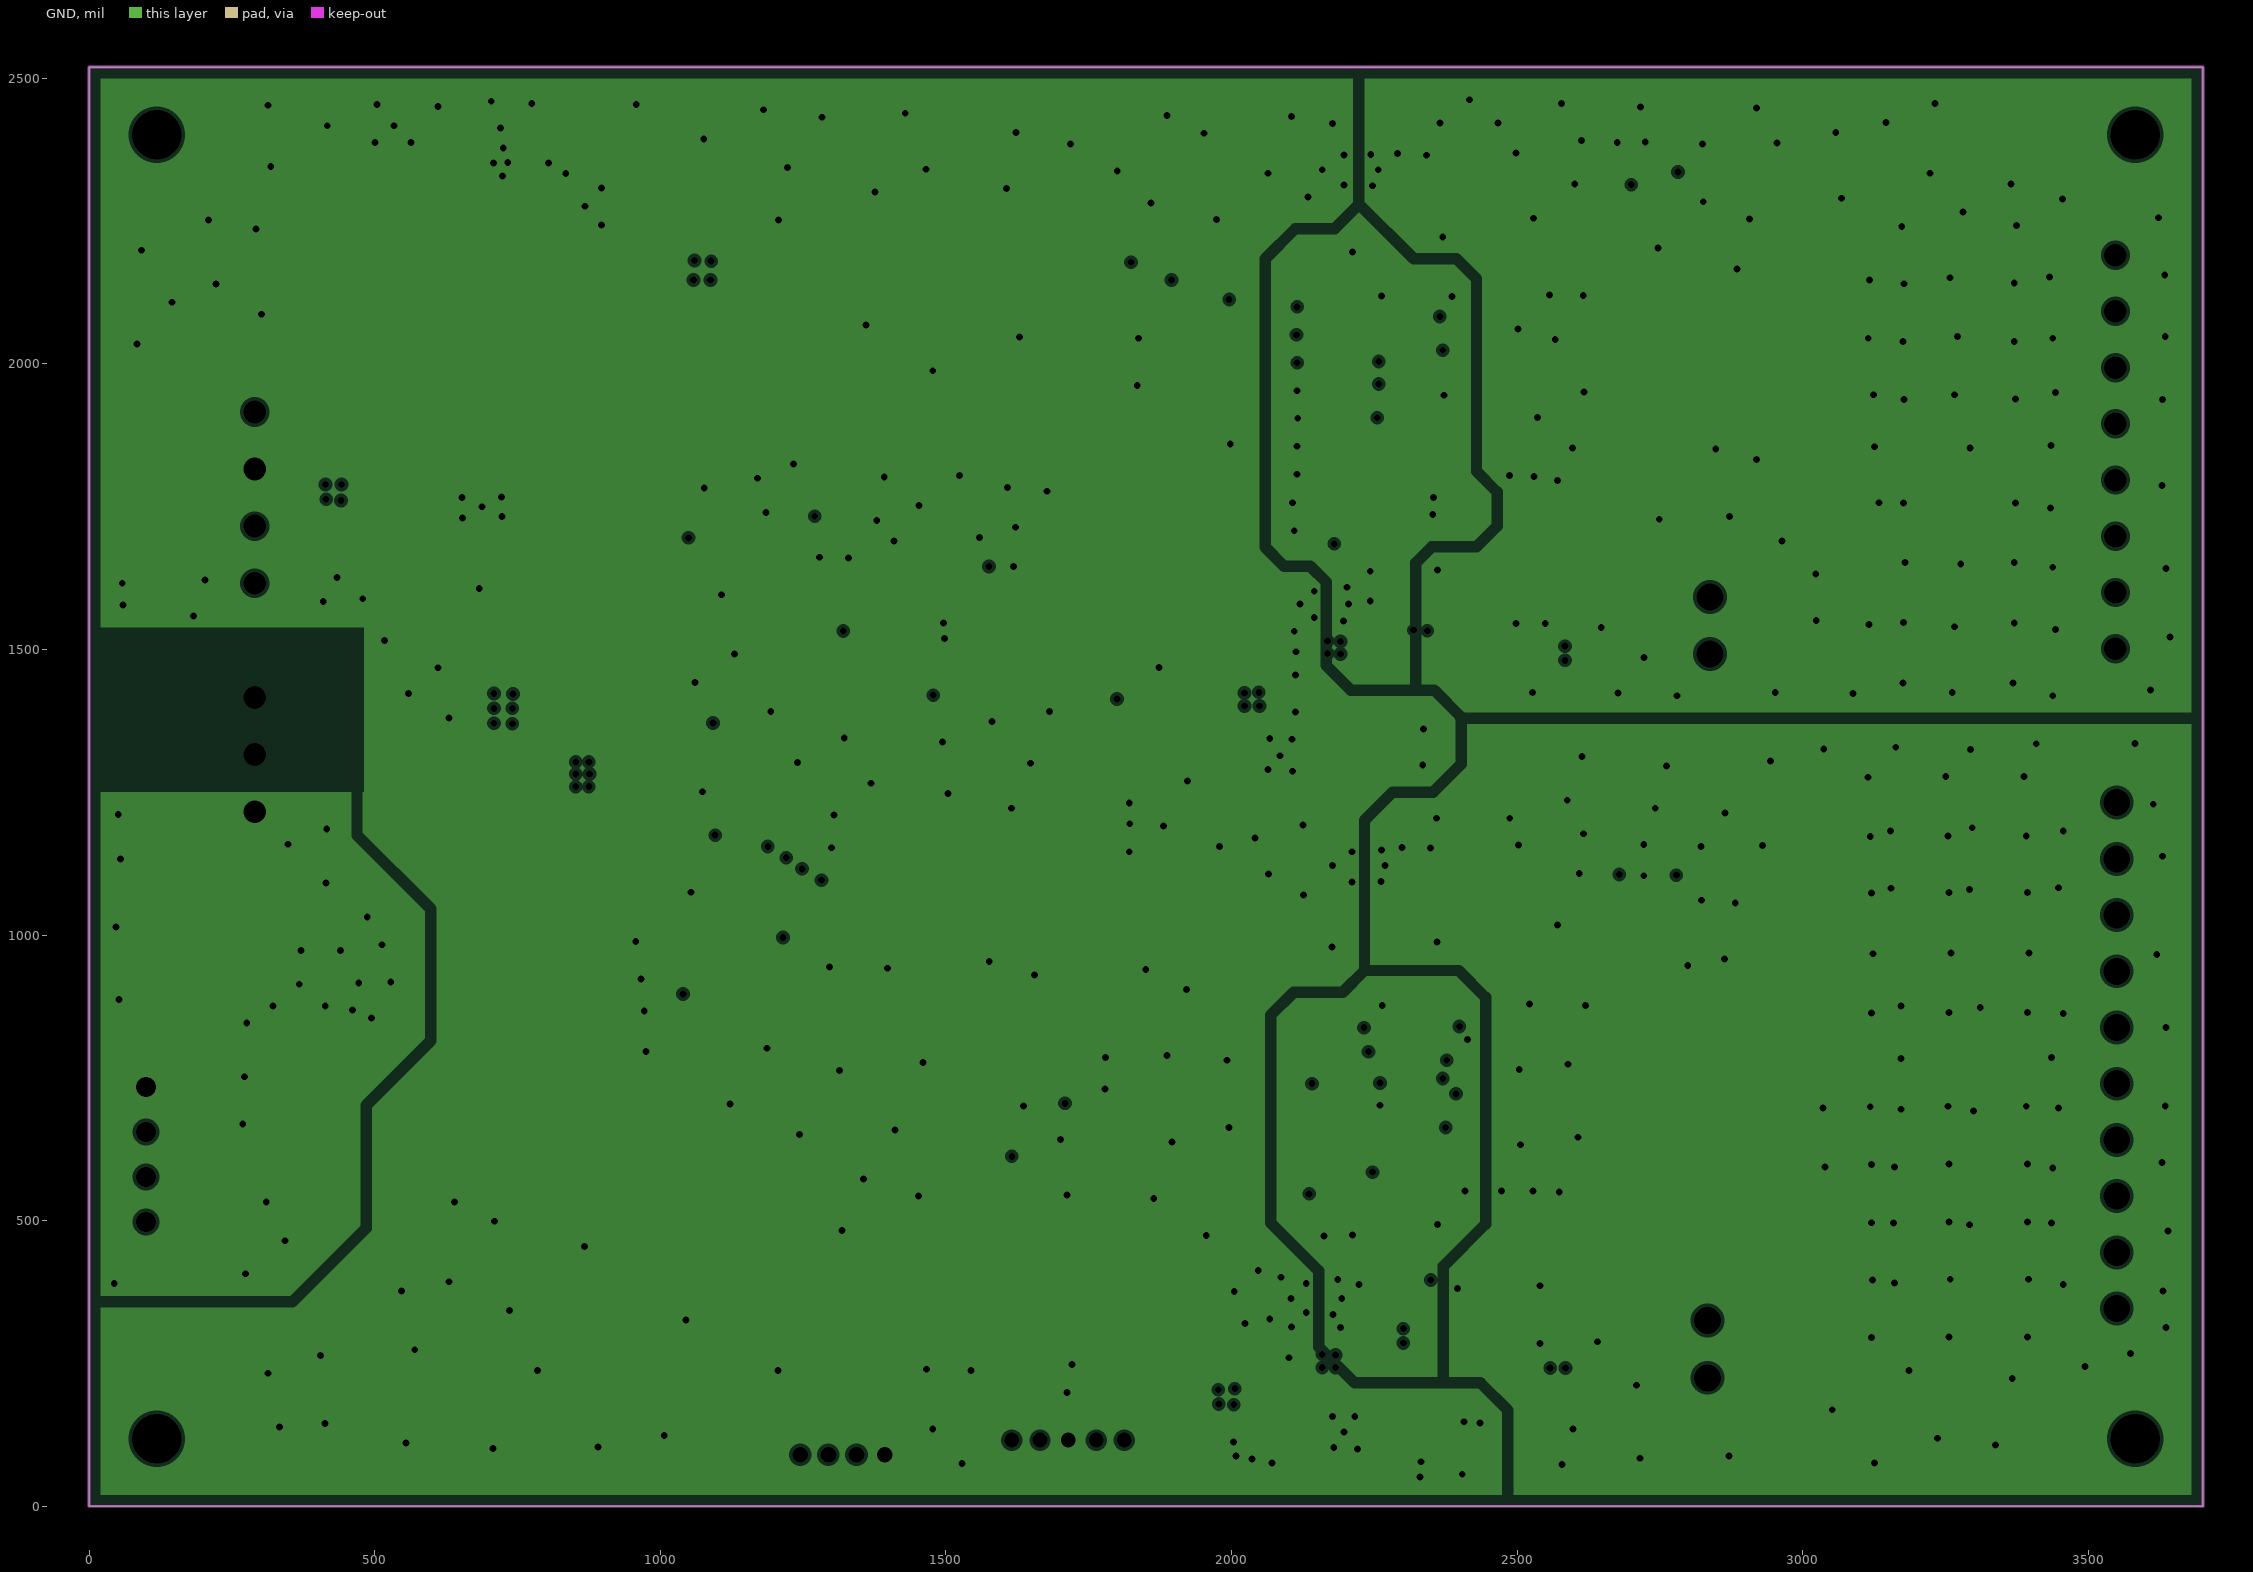
[diagram p0: GND, clearances drawn from the general rule]
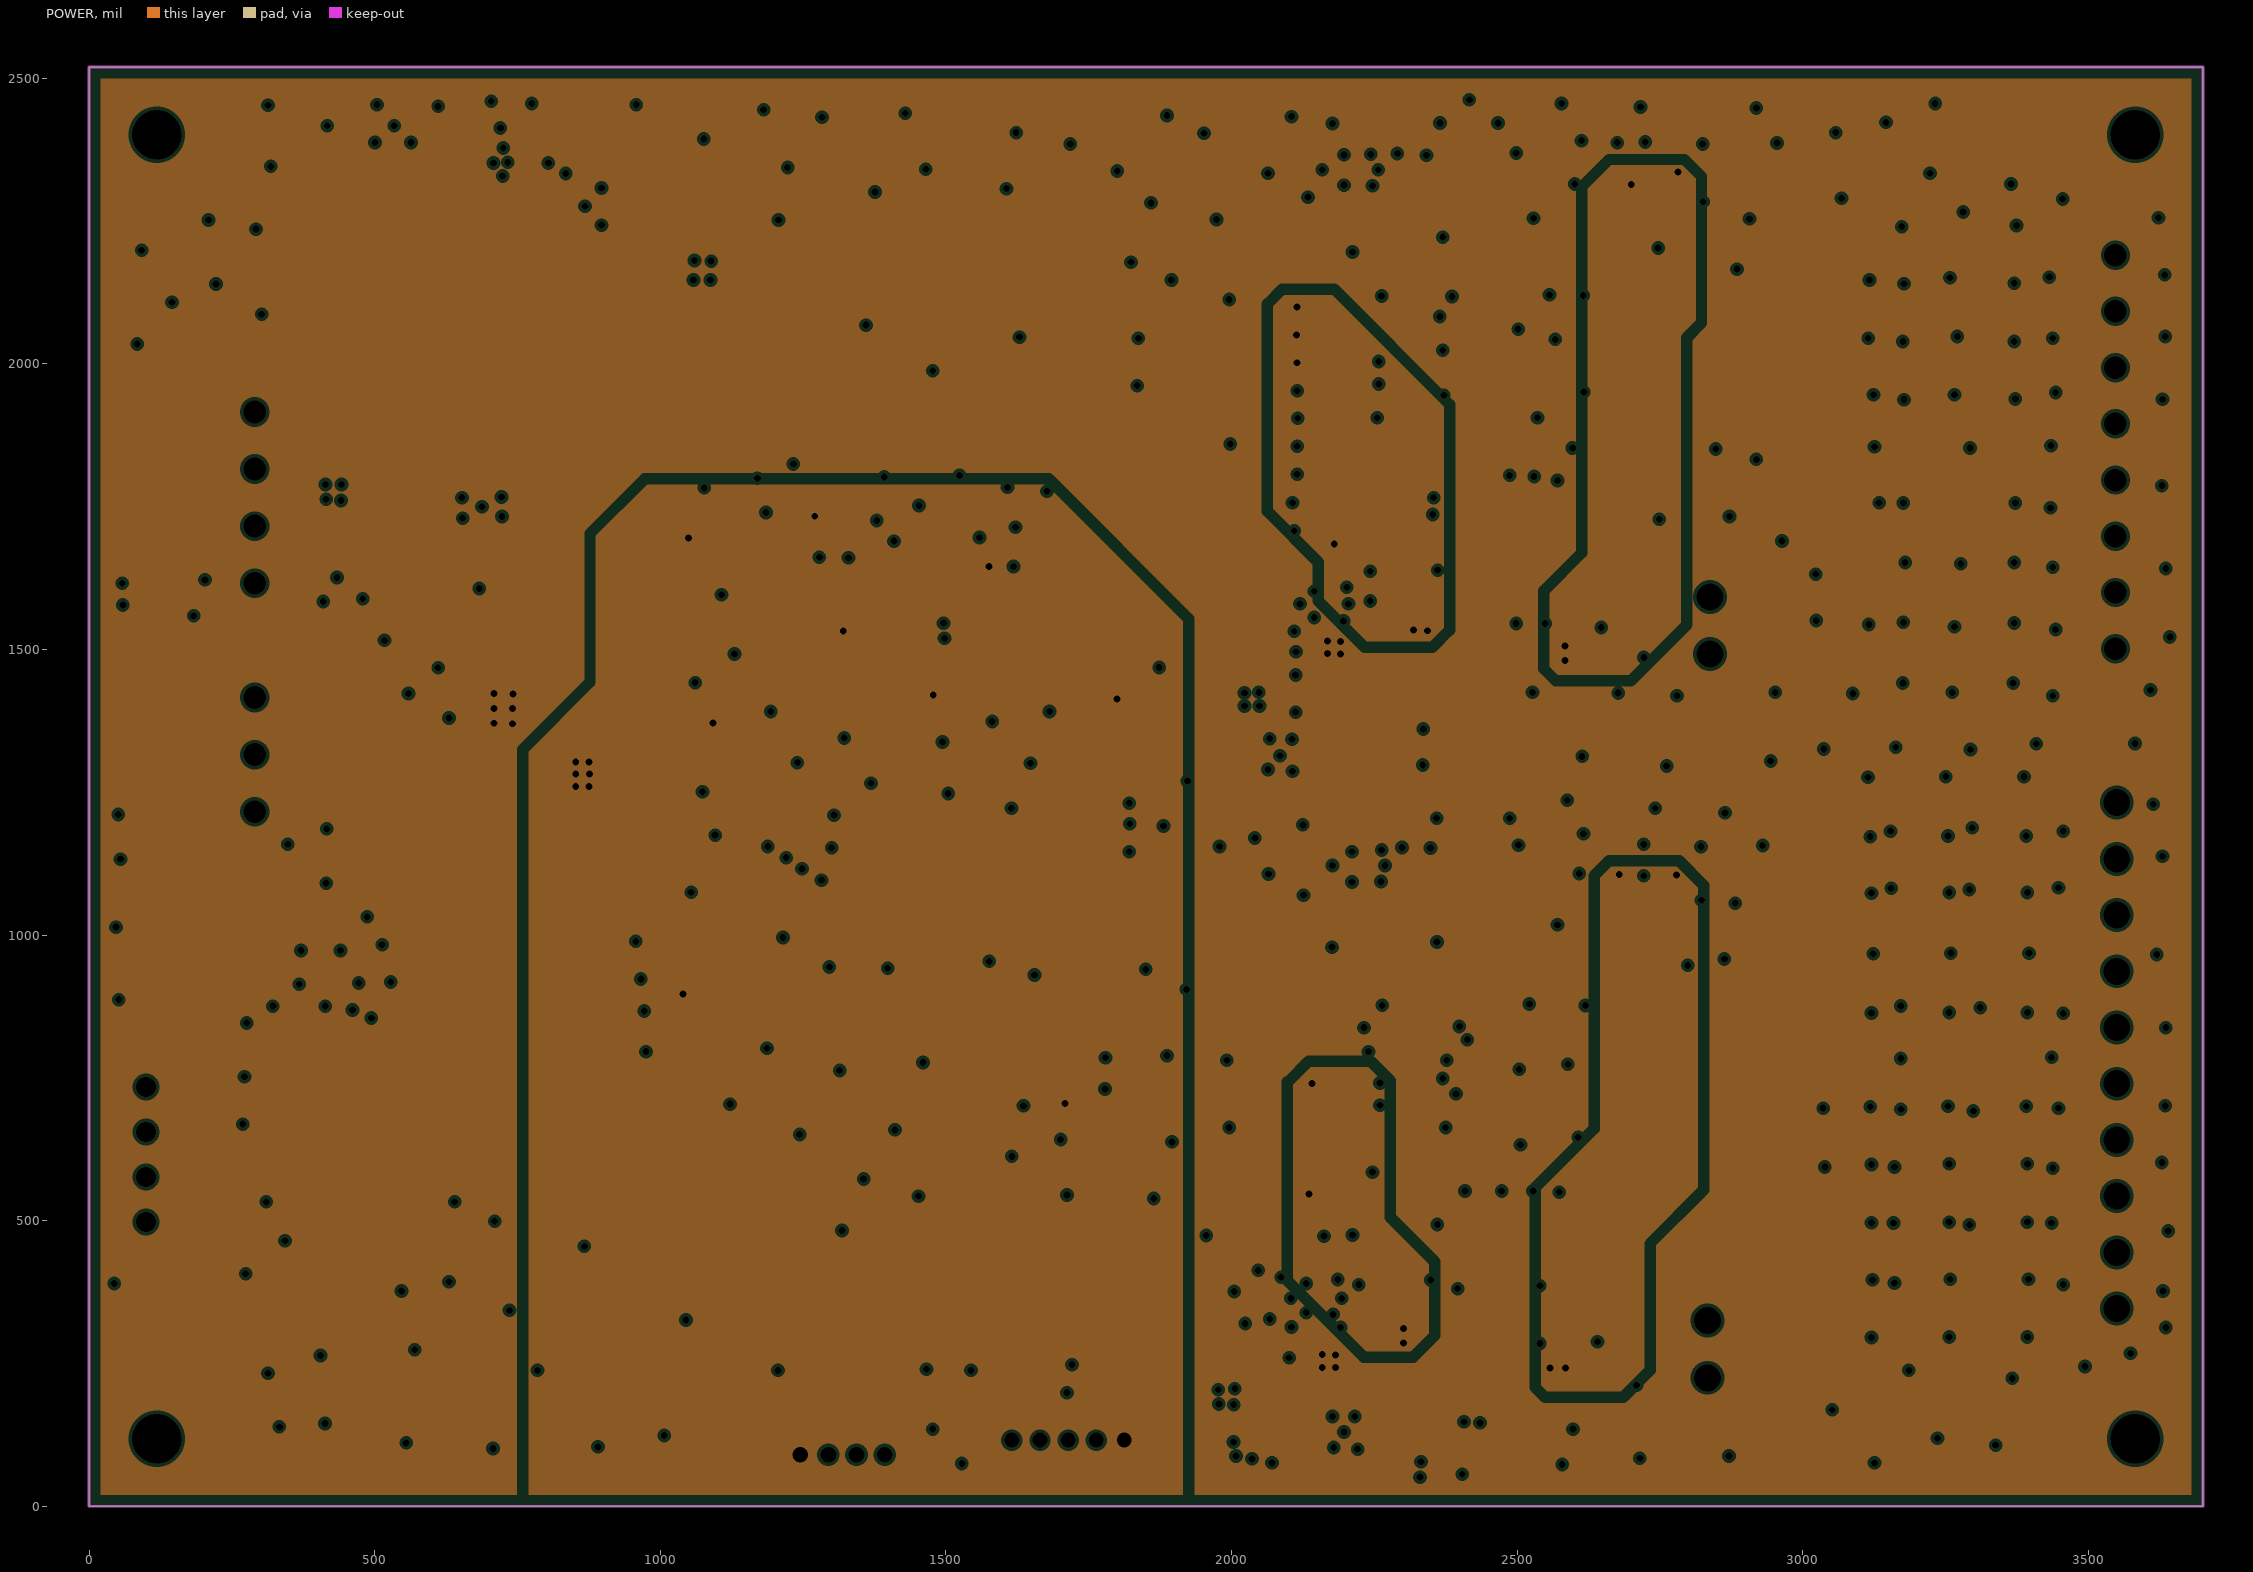
[diagram p1: POWER, clearances drawn from the general rule]
# Altium PCB MISC86293.PcbDoc (part 2 of 4)
## Footprints (in the part's own frame and the unit in brackets; to place one, negate y for a bottom-side part, rotate by r counter-clockwise, add the part's x,y. Pads: shape width x height; smd on the part's side, far side on the other; paste and mask are expansions set on the pad) (continued)
CAP-SMD_L3.2-W1.6 [mm]
  rect 1.2x1.4 smd: 1(-1.35,0) 2(1.35,0)
  silkscreen extent -1.6,-1.14 1.6,1.14
CONN-TH_4P-P1.25_WAFER-MX1.25-4PZZ [mm]
  rect 0.9x1.5 hole 0.7 paste+0 mask+0.05: 1(1.875,0) 2(0.625,0) 3(-0.625,0) 4(-1.875,0)
  silkscreen extent -3.43,-2.02 3.43,1.21
CONN-TH_5P-P1.25_XUNPU_WAFER-MX1.25-5PZZ [mm]
  rect 1x0.9 hole 0.65: 1(-2.5,0)
  round 1 hole 0.65: 2(-1.25,0) 3(0,0) 4(1.25,0) 5(2.5,0)
  silkscreen extent -4.07,-2.03 4.07,1.27
CONN-TH_A2001WV-4P [mm]
  round 1.5 hole 0.9 paste+0 mask+0.05: 1(3,0) 2(1,0) 3(-1,0) 4(-3,0)
  silkscreen extent -5,-1.8 5,2.7
CONN-TH_A2501WV-10P [mm]
  round 1.8 hole 1.2: 1(11.25,0) 2(8.75,0) 3(6.25,0) 4(3.75,0) 5(1.25,0) 6(-1.25,0) 7(-3.75,0) 8(-6.25,0) 9(-8.75,0) 10(-11.25,0)
  silkscreen extent -13.88,-2.38 13.82,3.5
CONN-TH_WF-1A254A8P [mm]
  round 1.6 hole 1: 1(-8.75,0) 2(-6.25,0) 3(-3.75,0) 4(-1.25,0) 5(1.25,0) 6(3.75,0) 7(6.25,0) 8(8.75,0)
  silkscreen extent -11.25,-2.35 11.25,3.55
CRYSTAL-SMD_4P-L3.2-W2.5-BL [mm]
  rect 1.4x1.2 smd: 1(-1.1,-0.85) 2(1.1,-0.85) 3(1.1,0.85) 4(-1.1,0.85)
  silkscreen extent -2.26,-1.91 2.03,1.68
HDR-TH_2P-P2.54-V-M [mm]
  rect 2x2 hole 1.2: 1(-1.27,0)
  round 2 hole 1.2: 2(1.27,0)
  silkscreen extent -2.54,-1.27 2.54,1.27
IND-SMD_L4.0-W4.0_FNR40XXS [mm]
  rect 1.6x3.9 smd: 1(-1.5,0) 2(1.5,0)
  silkscreen extent -2,-2.1 2,2.1
L0402 [mm]
  rect 0.79x0.54 smd paste-100 mask+0.051: 1(-0.545,0) 2(0.545,0)
  silkscreen extent -1.17,-0.5 1.17,0.5
L0603 [mm]
  rect 0.8x0.864 smd paste-100 mask+0.051: 1(-0.7,0) 2(0.7,0)
  silkscreen extent -1.42,-0.65 1.41,0.67
LED0603-RD [mm]
  rect 0.8x0.8 smd: 1(-0.799,0) 2(0.799,0)
  silkscreen extent -1.49,-0.75 1.39,0.76
LQFP-100_L14.0-W14.0-P0.50-LS16.0-BL [mm]
  oval 0.3x1.6 smd paste-100 mask+0.051: 1(-6,-7.55) 2(-5.5,-7.55) 3(-5,-7.55) 4(-4.5,-7.55) 5(-4,-7.55) 6(-3.5,-7.55) 7(-3,-7.55) 8(-2.5,-7.55) 9(-2,-7.55) 10(-1.5,-7.55) 11(-1,-7.55) 12(-0.5,-7.55) 13(0,-7.55) 14(0.5,-7.55) 15(1,-7.55) 16(1.5,-7.55) 17(2,-7.55) 18(2.5,-7.55) 19(3,-7.55) 20(3.5,-7.55) 21(4,-7.55) 22(4.5,-7.55) 23(5,-7.55) 24(5.5,-7.55) 25(6,-7.55) 51(6,7.55) 52(5.5,7.55) 53(5,7.55) 54(4.5,7.55) 55(4,7.55) 56(3.5,7.55) 57(3,7.55) 58(2.5,7.55) 59(2,7.55) 60(1.5,7.55) 61(1,7.55) 62(0.5,7.55) 63(0,7.55) 64(-0.5,7.55) 65(-1,7.55) 66(-1.5,7.55) 67(-2,7.55) 68(-2.5,7.55) 69(-3,7.55) 70(-3.5,7.55) 71(-4,7.55) 72(-4.5,7.55) 73(-5,7.55) 74(-5.5,7.55) 75(-6,7.55)
  oval 1.6x0.3 smd paste-100 mask+0.051: 26(7.55,-6) 27(7.55,-5.5) 28(7.55,-5) 29(7.55,-4.5) 30(7.55,-4) 31(7.55,-3.5) 32(7.55,-3) 33(7.55,-2.5) 34(7.55,-2) 35(7.55,-1.5) 36(7.55,-1) 37(7.55,-0.5) 38(7.55,0) 39(7.55,0.5) 40(7.55,1) 41(7.55,1.5) 42(7.55,2) 43(7.55,2.5) 44(7.55,3) 45(7.55,3.5) 46(7.55,4) 47(7.55,4.5) 48(7.55,5) 49(7.55,5.5) 50(7.55,6) 76(-7.55,6) 77(-7.55,5.5) 78(-7.55,5) 79(-7.55,4.5) 80(-7.55,4) 81(-7.55,3.5) 82(-7.55,3) 83(-7.55,2.5) 84(-7.55,2) 85(-7.55,1.5) 86(-7.55,1) 87(-7.55,0.5) 88(-7.55,0) 89(-7.55,-0.5) 90(-7.55,-1) 91(-7.55,-1.5) 92(-7.55,-2) 93(-7.55,-2.5) 94(-7.55,-3) 95(-7.55,-3.5) 96(-7.55,-4) 97(-7.55,-4.5) 98(-7.55,-5) 99(-7.55,-5.5) 100(-7.55,-6)
  silkscreen extent -7.03,-8 6.25,6.25
MSOP-10_L3.0-W3.0-P0.50-LS5.0-BL-EP [mm]
  oval 0.28x1.62 smd paste-100 mask+0.051: 1(-1,-2.11) 2(-0.5,-2.11) 3(0,-2.11) 4(0.5,-2.11) 5(1,-2.11) 6(1,2.11) 7(0.5,2.11) 8(0,2.11) 9(-0.5,2.11) 10(-1,2.11)
  rect 2.1x1.83 smd paste-100 mask+0.051: 11(0,0)
  silkscreen extent -1.84,-2.35 1.52,1.52
MSOP-12_L4.0-W3.0-P0.65-LS4.9-BL-EP [mm]
  rect 0.3x1.3 smd paste+0.051 mask+0: 1(-1.625,-2.375) 2(-0.975,-2.375) 3(-0.325,-2.375) 4(0.325,-2.375) 5(0.975,-2.375) 6(1.625,-2.375)
  rect 0.35x1.3 smd paste+0.051 mask+0: 7(1.625,2.375) 8(0.975,2.375) 9(0.325,2.375) 10(-0.325,2.375) 11(-0.975,2.375) 12(-1.625,2.375)
  rect 2.85x1.65 smd paste+0.051 mask+0: 13(0,-0.038)
  silkscreen extent -2.51,-2.3 1.98,1.45
PWRM-TH_WRA0512S-3WR2 [mil]
  round 70 hole 40 paste+2 mask+0: 1(-350,0) 2(-250,0) 3(-150,0) 5(50,0) 6(150,0) 7(250,0) 8(350,0)
  silkscreen extent -433,-276 433,98
R0402 [mm]
  rect 0.566x0.54 smd paste-100 mask+0.051: 1(-0.433,0) 2(0.433,0)
  silkscreen extent -0.94,-0.5 0.94,0.5
R0603 [mil]
  rect 31.75x34.02 smd paste-3937.01 mask+2: 1(-29.66,0) 2(29.66,0)
  silkscreen extent -55,-26 55,26
SMA_L4.3-W2.6-LS5.2-RD [mm]
  rect 2x2 smd: 1(-2.2,0) 2(2.2,0)
  silkscreen extent -2.98,-1.5 2.6,1.5
SOIC-8_L4.9-W3.9-P1.27-LS6.0-BL [mm]
  oval 0.588x2.045 smd: 1(-1.905,-2.772) 2(-0.635,-2.772) 3(0.635,-2.772) 4(1.905,-2.772) 5(1.905,2.772) 6(0.635,2.772) 7(-0.635,2.772) 8(-1.905,2.772)
  silkscreen extent -2.8,-2.92 2.53,1.52
SOT-23-3_L2.9-W1.3-P1.90-LS2.4-BR [mm]
  rect 1.25x0.7 smd: 1(1,-0.95) 2(1,0.95) 3(-1,0)
  silkscreen extent -0.73,-1.53 0.73,1.53
SOT-23-5_L3.0-W1.7-P0.95-LS2.8-BR [mm]
  rect 1.1x0.6 smd: 1(1.3,-0.95) 2(1.3,0) 3(1.3,0.95) 4(-1.3,0.95) 5(-1.3,-0.95)
  silkscreen extent -0.9,-1.78 1.65,1.55
SW-SMD_L3.9-W3.0-P4.45 [mm]
  rect 1.23x1.36 smd: 1(-2.185,0) 2(2.185,0)
  silkscreen extent -2.03,-1.62 2.25,1.62
TQFP-64_L10.0-W10.0-P0.50-LS12.0-BL [mm]
  oval 0.28x1.8 smd: 1(-3.75,-5.55) 2(-3.25,-5.55) 3(-2.75,-5.55) 4(-2.25,-5.55) 5(-1.75,-5.55) 6(-1.25,-5.55) 7(-0.75,-5.55) 8(-0.25,-5.55) 9(0.25,-5.55) 10(0.75,-5.55) 11(1.25,-5.55) 12(1.75,-5.55) 13(2.25,-5.55) 14(2.75,-5.55) 15(3.25,-5.55) 16(3.75,-5.55) 33(3.75,5.55) 34(3.25,5.55) 35(2.75,5.55) 36(2.25,5.55) 37(1.75,5.55) 38(1.25,5.55) 39(0.75,5.55) 40(0.25,5.55) 41(-0.25,5.55) 42(-0.75,5.55) 43(-1.25,5.55) 44(-1.75,5.55) 45(-2.25,5.55) 46(-2.75,5.55) 47(-3.25,5.55) 48(-3.75,5.55)
  oval 1.8x0.28 smd: 17(5.55,-3.75) 18(5.55,-3.25) 19(5.55,-2.75) 20(5.55,-2.25) 21(5.55,-1.75) 22(5.55,-1.25) 23(5.55,-0.75) 24(5.55,-0.25) 25(5.55,0.25) 26(5.55,0.75) 27(5.55,1.25) 28(5.55,1.75) 29(5.55,2.25) 30(5.55,2.75) 31(5.55,3.25) 32(5.55,3.75) 49(-5.55,3.75) 50(-5.55,3.25) 51(-5.55,2.75) 52(-5.55,2.25) 53(-5.55,1.75) 54(-5.55,1.25) 55(-5.55,0.75) 56(-5.55,0.25) 57(-5.55,-0.25) 58(-5.55,-0.75) 59(-5.55,-1.25) 60(-5.55,-1.75) 61(-5.55,-2.25) 62(-5.55,-2.75) 63(-5.55,-3.25) 64(-5.55,-3.75)
  silkscreen extent -5.4,-7.04 5,5
TQFP-64_L10.0-W10.0-P0.50-LS12.0-TL [mm]
  oval 1.8x0.28 smd paste-100 mask+0.051: 1(-5.55,3.75) 2(-5.55,3.25) 3(-5.55,2.75) 4(-5.55,2.25) 5(-5.55,1.75) 6(-5.55,1.25) 7(-5.55,0.75) 8(-5.55,0.25) 9(-5.55,-0.25) 10(-5.55,-0.75) 11(-5.55,-1.25) 12(-5.55,-1.75) 13(-5.55,-2.25) 14(-5.55,-2.75) 15(-5.55,-3.25) 16(-5.55,-3.75) 33(5.55,-3.75) 34(5.55,-3.25) 35(5.55,-2.75) 36(5.55,-2.25) 37(5.55,-1.75) 38(5.55,-1.25) 39(5.55,-0.75) 40(5.55,-0.25) 41(5.55,0.25) 42(5.55,0.75) 43(5.55,1.25) 44(5.55,1.75) 45(5.55,2.25) 46(5.55,2.75) 47(5.55,3.25) 48(5.55,3.75)
  oval 0.28x1.8 smd paste-100 mask+0.051: 17(-3.75,-5.55) 18(-3.25,-5.55) 19(-2.75,-5.55) 20(-2.25,-5.55) 21(-1.75,-5.55) 22(-1.25,-5.55) 23(-0.75,-5.55) 24(-0.25,-5.55) 25(0.25,-5.55) 26(0.75,-5.55) 27(1.25,-5.55) 28(1.75,-5.55) 29(2.25,-5.55) 30(2.75,-5.55) 31(3.25,-5.55) 32(3.75,-5.55) 49(3.75,5.55) 50(3.25,5.55) 51(2.75,5.55) 52(2.25,5.55) 53(1.75,5.55) 54(1.25,5.55) 55(0.75,5.55) 56(0.25,5.55) 57(-0.25,5.55) 58(-0.75,5.55) 59(-1.25,5.55) 60(-1.75,5.55) 61(-2.25,5.55) 62(-2.75,5.55) 63(-3.25,5.55) 64(-3.75,5.55)
  silkscreen extent -5.95,-5 5,5
X1-DFN1006-2_L1.0-W0.6-BI [mil]
  rect 31.11x25.51 smd paste-3937.01 mask+2: 1(-21.46,0) 2(21.46,0)
  silkscreen extent -46,-22 46,22

## Part data
C3 C6 C42 C71: library part CL10A106MA8NRNC
C7: library part CL10A106KP8NNNC
C8 C10: library part CL05A105KA5NQNC
C9: library part CA45-A-16V-22uF-K
C23: library part CL05B103KB5NNNC
C24 C25 C27 C29 C30 C32 C34 C36 C38 C40 C53 C54 C56 C58 C59 C61 C63 C65 C67 C69: library part GRM155Z71A105KE01D
C26: library part GRM31CR61A107ME05L
C28 C31 C33 C35 C37 C39 C41 C43 C57 C60 C62 C64 C66 C68 C70 C72: library part CL05B104KB54PNC
C44 C45 C46 C47 C48 C49 C50 C51: library part 0402B472K500NT
C52: library part CC0402KRX7R9BB152
C55: library part CL31A226KAHNNNE
C73 C74 C75 C76 C77 C78 C79 C80 C81 C82 C83 C84 C85 C86 C87 C88 C89 C90 C91 C92: library part 0402CG470J500NT
C93 C94 C98 C99 C100 C101 C102 C103 C104: library part CC0402KRX7R7BB104
C95: library part CC0402KRX5R6BB105
C96 C106: library part 0603B225K160NT
C97: library part 0603X106K100NT
C105 C107: library part AC0402JRNPO9BN120
C108 C109: library part GRM31CR61A107MEA8L
C110: library part GRM31CR61A476ME15L
C111: library part GRM31CR71A226KE15L
C112 C113 C115 C117 C118: library part GRM188Z71C475KE21D
C114 C116 C119: library part GRM188R71A474KA61D
C120: library part GRM188Z71A106KA73D
L1: library part FNR4030S4R7MT
R1: library part 0603WAF1001T5E
R3 R5 R11 R12 R13 R14 R15 R16 R17 R18 R30 R31 R32 R33 R55 R56: library part RC0402FR-0710KL
R4: library part 0402WGF4022TCE
R6 R7 R58 R59: library part 0402WGJ0000TCE
R8: library part FRC0402F3923TS
R9 R28 R54: library part 0402WGF0000TCE
R10 R29: library part RC0402FR-07100KL
R19 R20 R21 R22 R23 R24 R25 R26: library part 0402WGF4991TCE
R27: library part SC0402F1004F2ANRH
R34 R36 R38 R40 R42 R44 R46 R48 R50 R52: library part AC0402FR-0722K1L
R35 R37 R39 R41 R43 R45 R47 R49 R51 R53: library part 0402WGF1002TCE
R57: library part 0402WGF470JTCE
R60 R62: library part 0603WAD3322T5E
R61: library part 0603WAF4992T5E
U5: library part _122M31
X1: library part X32258MOB4SI

## Free pads (board coordinates)
  round 157.48 hole 86.61: 0(118.11,118.11) 1(3582.68,118.11) 2(3582.68,2401.57) 3(118.11,2401.57)
  round 39.37 smd mask+39.37: MARK(108,269) MARK(3397,2413)

## Via types
v1: diameter 20, hole 12, Top Layer to Bottom Layer, 581 vias

## Nets (pads, with @x,y where several pads share a name; then routed paths per layer and width w, separated by ;. In a path a pad name is that pad's centre, name@x,y a point inside that pad or via, vN(x,y) a via of type N, cw(c..) or ccw(c..) an arc to the next point about the centre after c; other vN are vias at no path point)
ADS_CLK: U8.37 U9.37 | length 1419.9
  Top Layer w6: U8.37@2308.98,2023.9 v1(2369.9,2023.9) ; U9.37@2312.98,780.9 v1@2373.1,780.9
  Bottom Layer w6: v1(2369.9,2023.9) 2441,1952.8 2441,917 2377,853 v1(2377,781)
ADS_SPI_CLK: U8.40 U9.40 U10.30 | length 3678.4
  Top Layer w6: U10.30@1141.24,1332.48 1056.52,1332.48 953,1436 953,1833 1268,2148 v1@1894,2148 ; v1(2257.84,1964.84) U8.40@2308.98,1964.84 ; U9.40@2312.98,721.84 v1@2392.84,721.84
  Bottom Layer w6: v1(1895,2147) 2063,1979 2243.68,1979 v1(2257.84,1964.84) 2321.16,1964.84 2400,1886 2400,943 2331,874 2331,756 2365,722 v1(2393,722)
ADS_SPI_DI/MCU_DO: U8.34 U9.34 U10.32 | length 3769.9
  Top Layer w6: U10.32@1141.24,1293.11 1021.89,1293.11 904,1411 904,1859 1251,2206 1875,2206 1922,2159 2184,2159 2260,2083 U8.34@2300,2083 ; U8.34@2308.98,2082.95 v1(2364.95,2082.95) ; U9.34@2312.98,839.95 v1@2392.05,839.95
  Bottom Layer w6: v1(2364.95,2082.95) 2463,1984.9 2463,904 v1(2399,840)
ADS_SPI_DO/MCU_DI: U8.43 U9.43 U10.31 | length 3767.3
  Top Layer w6: U10.31@1141.24,1312.8 1038.2,1312.8 927,1424 927,1844 1262,2179 1820,2179 v1@1823,2176 ; v1(2255.21,1905.79) U8.43@2308.98,1905.79 ; U9.43@2312.98,662.79 v1@2370.21,662.79
  Bottom Layer w6: v1(1824,2178) 2071,1931 2210,1931 2235.21,1905.79 v1(2255.21,1905.79) 2340.21,1905.79 2380,1866 2380,953 2315,888 2315,723 v1(2375,663)